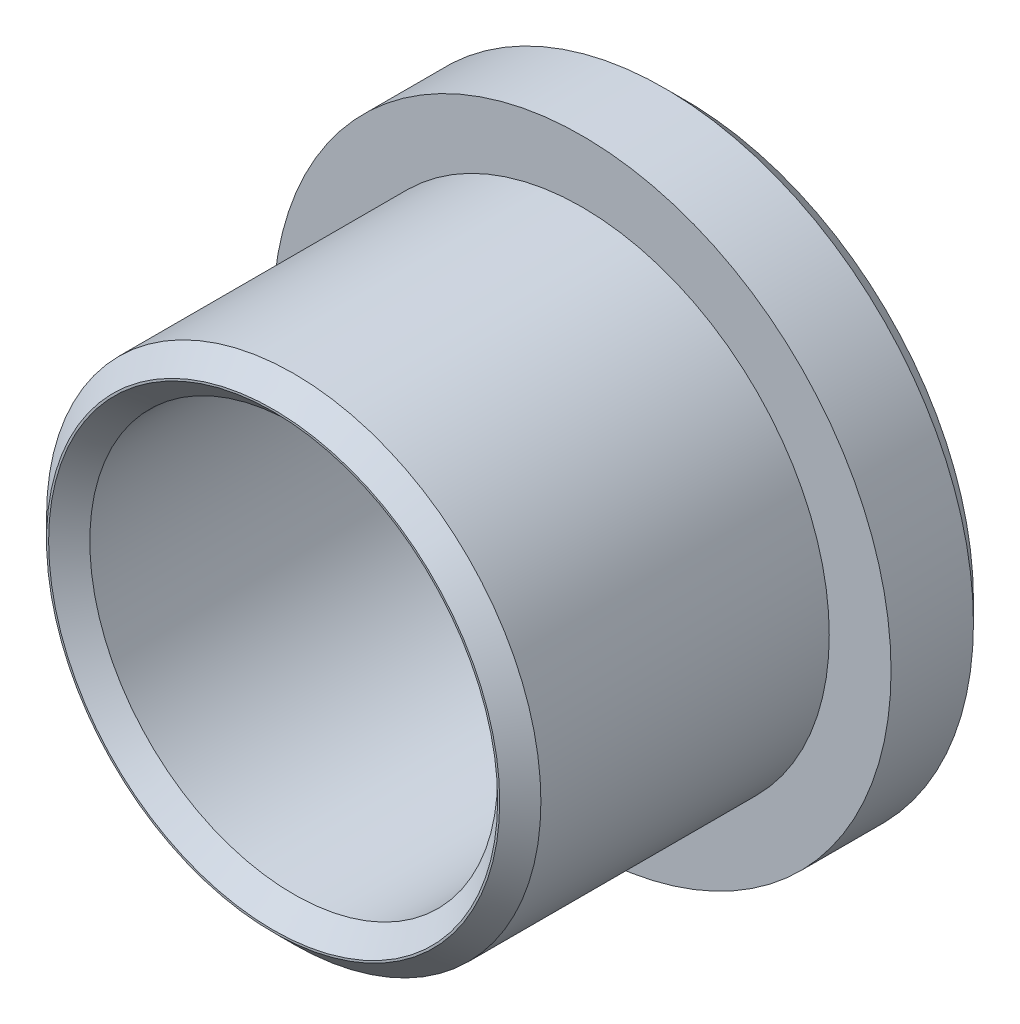
SolidWorks part; units mm, degrees
ref_plane "Front Plane" through (0, 0, 0) normal (0, 0, 1) x (1, 0, 0)
ref_plane "Top Plane" through (0, 0, 0) normal (0, 1, 0) x (1, 0, 0)
ref_plane "Right Plane" through (0, 0, 0) normal (1, 0, 0) x (0, 0, -1)
sketch "Sketch1" plane through (0, 0, 0) normal (0, 0, 1) x (1, 0, 0)
  circle A0 centre (0, 0) radius 15
  circle A1 centre (0, 0) radius 9.9
extrude "Boss-Extrude1" add sketch "Sketch1" along normal blind 5
sketch "Sketch2" plane through (0, 0, 5) normal (0, 0, 1) x (1, 0, 0)
  circle A0 centre (0, 0) radius 9.9
  circle A1 centre (0, 0) radius 12
extrude "Boss-Extrude2" add sketch "Sketch2" along normal blind 15
chamfer "Chamfer1" distance 1 distance2 1 3 edges at (15, 0, 0) (12, 0, 20) (9.9, 0, 20)
